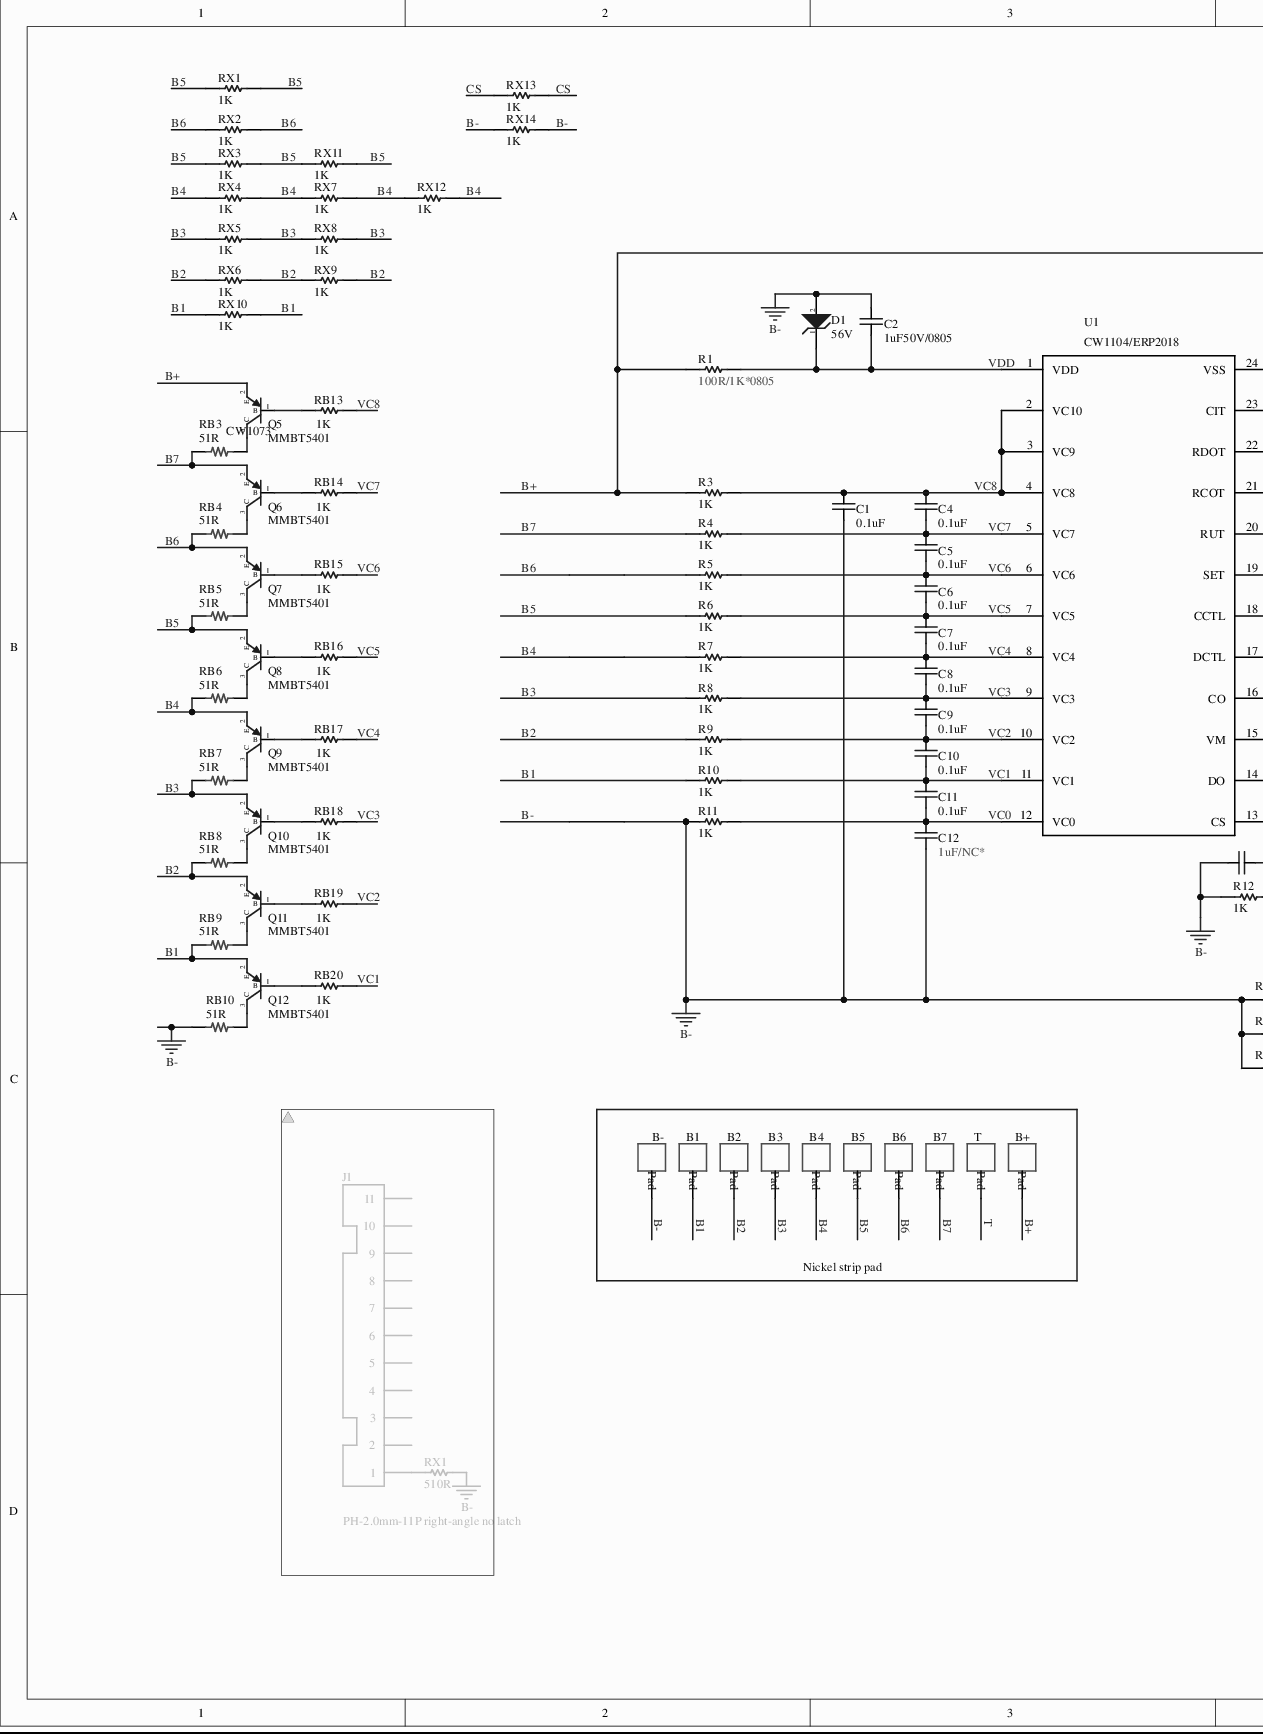
[diagram p0: MISC84401-5.SchDoc, left]
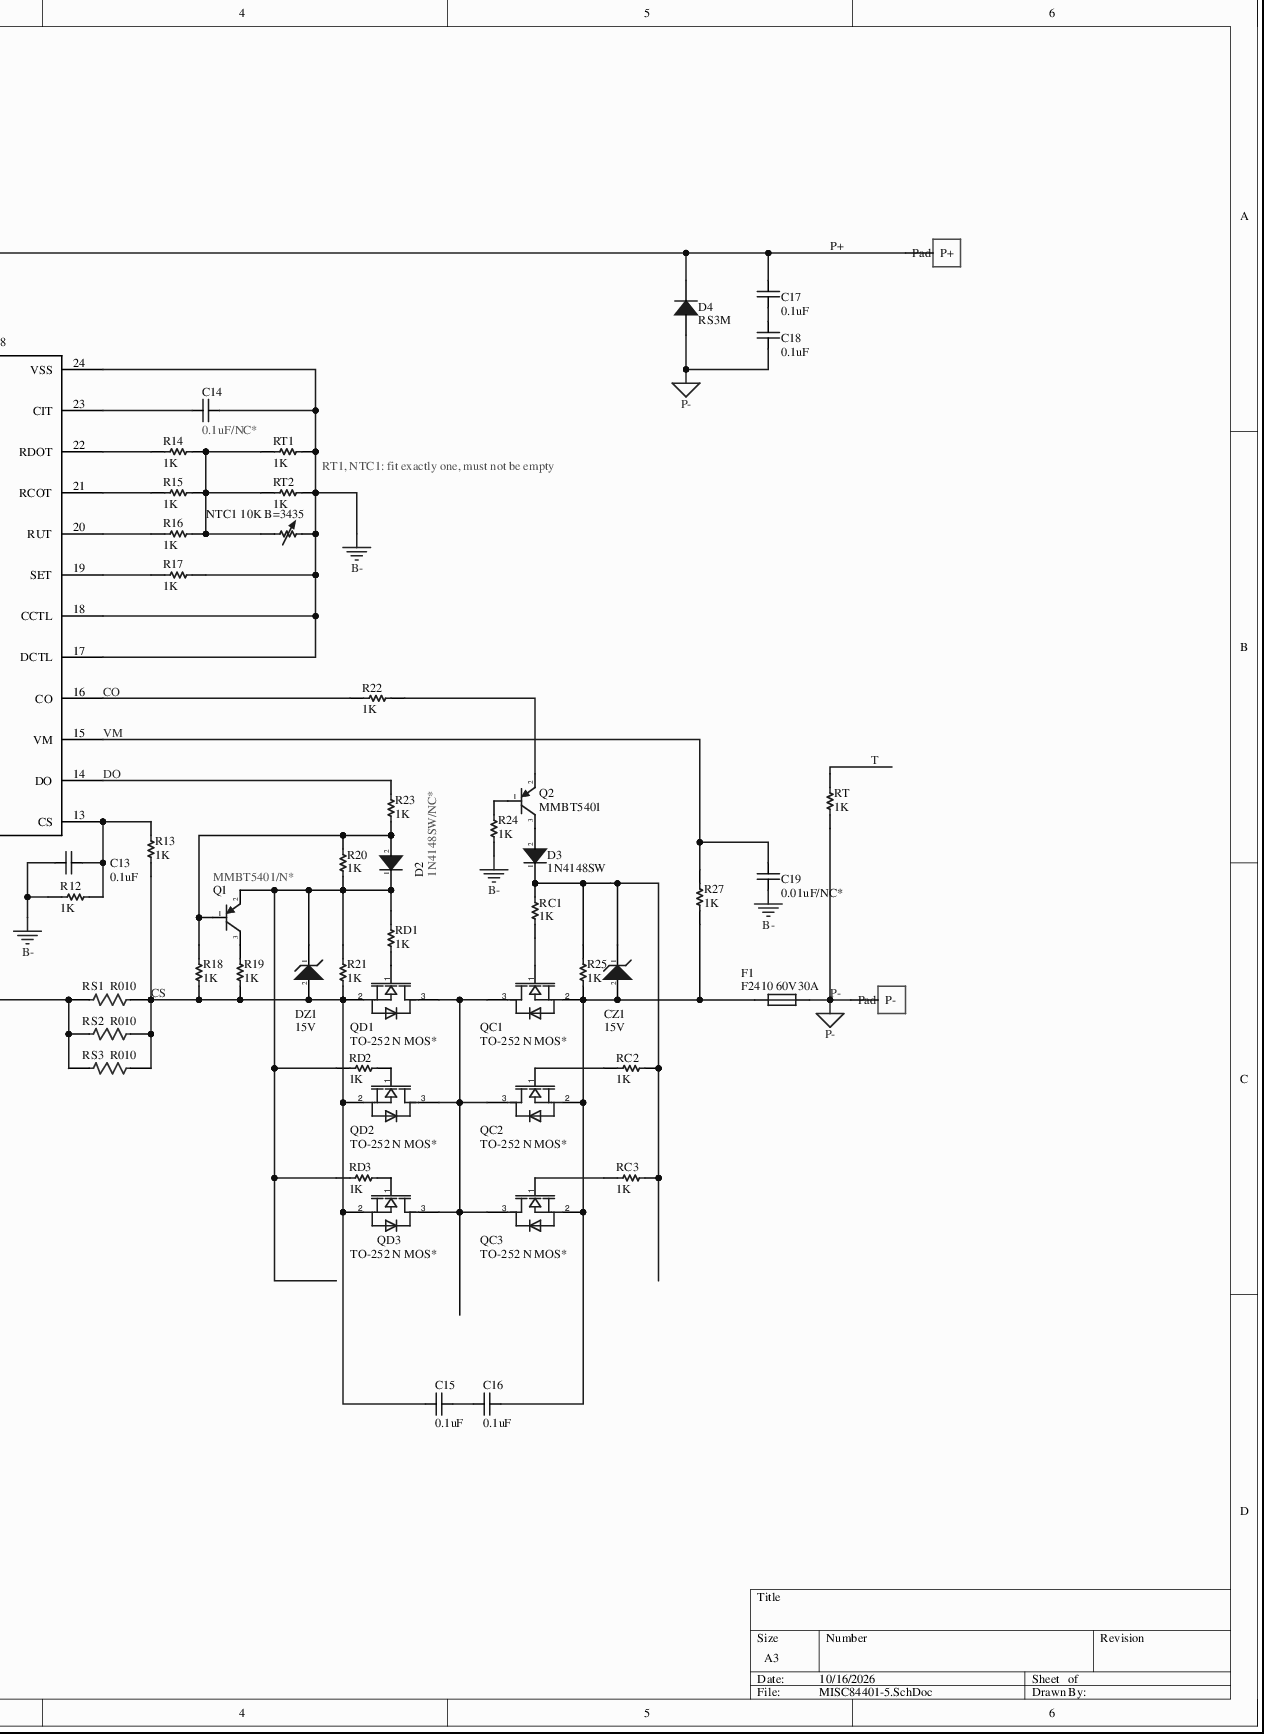
[diagram p1: MISC84401-5.SchDoc, right]
# Altium project MISC84401-3.PrjPcb
1 sheet, 124 parts. Net scope: global (net labels, ports and power ports of the same name join across sheets).
Board file: MISC84401.PcbDoc

## Sheet MISC84401-5.SchDoc
size 449 x 320 mm; SheetNumber: 1; SheetTotal: 1

### Parts
(Parts that share a designator on the sheet are numbered #1, #2 ... from top to bottom, then left to right.)
B1  Pad  [Pad10X8mm]
B2  Pad  [Pad10X8mm]
B3  Pad  [Pad10X8mm]
B4  Pad  [Pad10X8mm]
B5  Pad  [Pad10X8mm]
B6  Pad  [Pad10X8mm]
B7  Pad  [Pad10X8mm]
B+  Pad  [Pad10X8mm]
B-  Pad  [Pad10X8mm]
C1  0.1uF  [C0603A]
C2  1uF50V/0805  [C0805A]
C4  0.1uF  [C0603A]
C5  0.1uF  [C0603A]
C6  0.1uF  [C0603A]
C7  0.1uF  [C0603A]
C8  0.1uF  [C0603A]
C9  0.1uF  [C0603A]
C10  0.1uF  [C0603A]
C11  0.1uF  [C0603A]
C12  1uF/NC*  [C0603A]
C13  0.1uF  [C0603A]
C14  0.1uF/NC*  [C0603A]
C15  0.1uF  [C0603A]
C16  0.1uF  [C0603A]
C17  0.1uF  [C0603A]
C18  0.1uF  [C0603A]
C19  0.01uF/NC*  [C0603A]
CZ1  15V  [SOD323]
D1  56V  [SOD323]
D2  1N4148SW/NC*  [SOD323]
D3  1N4148SW  [SOD323]
D4  RS3M  [SMB(DO-214AA)]
DZ1  15V  [SOD323]
F1  F2410 60V30A  [F2410]
J1  PH-2.0mm-11P right-angle no latch  [PH-2.0mm11P弯脚不带扣]  (masked out: inside a compile mask, not in the netlist)
NTC1  10K B=3435  [RT2.3X1.2-2]
P+  Pad  [Pad10X8mm]
P-  Pad  [Pad10X8mm]
Q1  MMBT5401/N*  [SOT23-3]
Q2  MMBT5401  [SOT23-3]
Q5  MMBT5401  [SOT23-3]
Q6  MMBT5401  [SOT23-3]
Q7  MMBT5401  [SOT23-3]
Q8  MMBT5401  [SOT23-3]
Q9  MMBT5401  [SOT23-3]
Q10  MMBT5401  [SOT23-3]
Q11  MMBT5401  [SOT23-3]
Q12  MMBT5401  [SOT23-3]
QC1  TO-252 N MOS*  [TO-252]
QC2  TO-252 N MOS*  [TO-252]
QC3  TO-252 N MOS*  [TO-252]
QD1  TO-252 N MOS*  [TO-252]
QD2  TO-252 N MOS*  [TO-252]
QD3  TO-252 N MOS*  [TO-252]
R1  100R/1K*0805  [R0805A]
R3  1K  [R0603A]
R4  1K  [R0603A]
R5  1K  [R0603A]
R6  1K  [R0603A]
R7  1K  [R0603A]
R8  1K  [R0603A]
R9  1K  [R0603A]
R10  1K  [R0603A]
R11  1K  [R0603A]
R12  1K  [R0603A]
R13  1K  [R0603A]
R14  1K  [R0603A]
R15  1K  [R0603A]
R16  1K  [R0603A]
R17  1K  [R0603A]
R18  1K  [R0603A]
R19  1K  [R0603A]
R20  1K  [R0603A]
R21  1K  [R0603A]
R22  1K  [R0603A]
R23  1K  [R0603A]
R24  1K  [R0603A]
R25  1K  [R0603A]
R27  1K  [R0603A]
RB3  51R  [R1206A]
RB4  51R  [R1206A]
RB5  51R  [R1206A]
RB6  51R  [R1206A]
RB7  51R  [R1206A]
RB8  51R  [R1206A]
RB9  51R  [R1206A]
RB10  51R  [R1206A]
RB13  1K  [R0603A]
RB14  1K  [R0603A]
RB15  1K  [R0603A]
RB16  1K  [R0603A]
RB17  1K  [R0603A]
RB18  1K  [R0603A]
RB19  1K  [R0603A]
RB20  1K  [R0603A]
RC1  1K  [R0603A]
RC2  1K  [R0603A]
RC3  1K  [R0603A]
RD1  1K  [R0603A]
RD2  1K  [R0603A]
RD3  1K  [R0603A]
RS1  R010  [R2512L]
RS2  R010  [R2512L]
RS3  R010  [R2512L]
RT  1K  [R0603A]
RT1  1K  [R0603A]
RT2  1K  [R0603A]
RX1#1  1K  [R1206A]
RX1#2  510R  [R0805A]  (masked out: inside a compile mask, not in the netlist)
RX2  1K  [R1206A]
RX3  1K  [R1206A]
RX4  1K  [R1206A]
RX5  1K  [R1206A]
RX6  1K  [R1206A]
RX7  1K  [R1206A]
RX8  1K  [R1206A]
RX9  1K  [R1206A]
RX10  1K  [R1206A]
RX11  1K  [R1206A]
RX12  1K  [R1206A]
RX13  1K  [R0805A]
RX14  1K  [R0805A]
T  Pad  [Pad10X8mm]
U1  CW1104/ERP2018  [TSSOP-24(pin间距0.635mm)]

### Blocks framed on the sheet
Nickel strip pad: B1-B7 B+ B- T

### Nets
B-: B-.1 C1.1 C2.1 C12.1 C13.1 C14.1 C19.2 D1.2(K) NTC1.2 R11.1 R12.1 R17.2 R24.2 RB10.1 RS1.1 RS2.1 RS3.1 RT1.2 RT2.2 RX14.1 RX14.2 U1.17(DCTL) U1.18(CCTL) U1.24(VSS)
P-: C18.1 D4.2(K) F1.2 P-.1 RT.1
B1: B1.1 Q12.2(E) R10.1 RB9.1 RX10.1 RX10.2
B2: B2.1 Q11.2(E) R9.1 RB8.1 RX6.1 RX6.2 RX9.1 RX9.2
B3: B3.1 Q10.2(E) R8.1 RB7.1 RX5.1 RX5.2 RX8.1 RX8.2
B4: B4.1 Q9.2(E) R7.1 RB6.1 RX4.1 RX4.2 RX7.1 RX7.2 RX12.1 RX12.2
B5: B5.1 Q8.2(E) R6.1 RB5.1 RX1#1.1 RX1#1.2 RX3.1 RX3.2 RX11.1 RX11.2
B6: B6.1 Q7.2(E) R5.1 RB4.1 RX2.1 RX2.2
B7: B7.1 Q6.2(E) R4.1 RB3.1
B+: B+.1 C17.2 D4.1(A) P+.1 Q5.2(E) R1.1 R3.1
CO: R22.1 U1.16(CO)
CS: C15.2 DZ1.2(K) QD1.2(S) QD2.2(S) QD3.2(S) R13.2 R18.2 R19.2 R21.2 RS1.2 RS2.2 RS3.2 RX13.1 RX13.2
DO: R23.1 U1.14(DO)
T: RT.2 T.1
VC0: C11.1 C12.2 R11.2 U1.12(VC0)
VC1: C10.1 C11.2 R10.2 RB20.2 U1.11(VC1)
VC2: C9.1 C10.2 R9.2 RB19.2 U1.10(VC2)
VC3: C8.1 C9.2 R8.2 RB18.2 U1.9(VC3)
VC4: C7.1 C8.2 R7.2 RB17.2 U1.8(VC4)
VC5: C6.1 C7.2 R6.2 RB16.2 U1.7(VC5)
VC6: C5.1 C6.2 R5.2 RB15.2 U1.6(VC6)
VC7: C4.1 C5.2 R4.2 RB14.2 U1.5(VC7)
VC8: C1.2 C4.2 R3.2 RB13.2 U1.2(VC10) U1.3(VC9) U1.4(VC8)
VDD: C2.2 D1.1(A) R1.2 U1.1(VDD)
VM: C19.1 R27.2 U1.15(VM)
NetC13_2: C13.2 R12.2 R13.1 U1.13(CS)
NetC14_2: C14.2 U1.23(CIT)
NetC15_1: C15.1 C16.2
NetC16_1: C16.1 CZ1.2(K) F1.1 QC1.2(S) QC2.2(S) QC3.2(S) R25.2 R27.1
NetC17_1: C17.1 C18.2
NetCZ1_1: CZ1.1(A) D3.1(A) R25.1 RC1.2 RC2.1 RC3.1
NetD2_1: D2.1(A) DZ1.1(A) Q1.2(E) R20.2 R21.1 RD1.2 RD2.2 RD3.2
NetD2_2: D2.2(K) Q1.1(B) R18.1 R20.1 R23.2
NetD3_2: D3.2(K) Q2.3(C)
NetNTC1_1: NTC1.1 R14.2 R15.2 R16.2 RT1.1 RT2.1
NetQ1_3: Q1.3(C) R19.1
NetQ2_1: Q2.1(B) R24.1
NetQ2_2: Q2.2(E) R22.2
NetQ5_1: Q5.1(B) RB13.1
NetQ5_3: Q5.3(C) RB3.2
NetQ6_1: Q6.1(B) RB14.1
NetQ6_3: Q6.3(C) RB4.2
NetQ7_1: Q7.1(B) RB15.1
NetQ7_3: Q7.3(C) RB5.2
NetQ8_1: Q8.1(B) RB16.1
NetQ8_3: Q8.3(C) RB6.2
NetQ9_1: Q9.1(B) RB17.1
NetQ9_3: Q9.3(C) RB7.2
NetQ10_1: Q10.1(B) RB18.1
NetQ10_3: Q10.3(C) RB8.2
NetQ11_1: Q11.1(B) RB19.1
NetQ11_3: Q11.3(C) RB9.2
NetQ12_1: Q12.1(B) RB20.1
NetQ12_3: Q12.3(C) RB10.2
NetQC1_1: QC1.1(G) RC1.1
NetQC1_3: QC1.3(D) QC2.3(D) QC3.3(D) QD1.3(D) QD2.3(D) QD3.3(D)
NetQC2_1: QC2.1(G) RC2.2
NetQC3_1: QC3.1(G) RC3.2
NetQD1_1: QD1.1(G) RD1.1
NetQD2_1: QD2.1(G) RD2.1
NetQD3_1: QD3.1(G) RD3.1
NetR14_1: R14.1 U1.22(RDOT)
NetR15_1: R15.1 U1.21(RCOT)
NetR16_1: R16.1 U1.20(RUT)
NetR17_1: R17.1 U1.19(SET)

### Notes on the sheet
- P+
- (near Q5) CW1073
- RT1, NTC1: fit exactly one, must not be empty

### Library data of the parts
B1-B7 B+ B- P+ P- T = Pad: Connection pad (non-through-hole)
C1 C2 C4-C19 = CAP: SMD capacitor
CZ1 D1 DZ1 = 5V6: SMD Zener diode
D2 D3 = 1N4148SW: SMD diode
D4 = RS3M: SMD diode
F1 = FUSE
J1 = PH-2.0mm-11P弯脚不带扣: Right-angle connector without latch
NTC1 = NTC: SMD thermistor
Q1 Q2 Q5-Q12 = MMBT5401: SMD transistor
QC1-QC3 QD1-QD3 = N MOS*: SMD MOS
R1 R3-R25 R27 RB13-RB20 RC1-RC3 RD1-RD3 RT RT1 RT2 RX1#1 RX1#2 RX2-RX14 = RES: SMD resistor
RB3-RB10 = RES3: Alloy SMD resistor
RS1-RS3 = RES2: SMD alloy resistor
U1 = CW1104*: Cellwise 7-10S battery protection IC